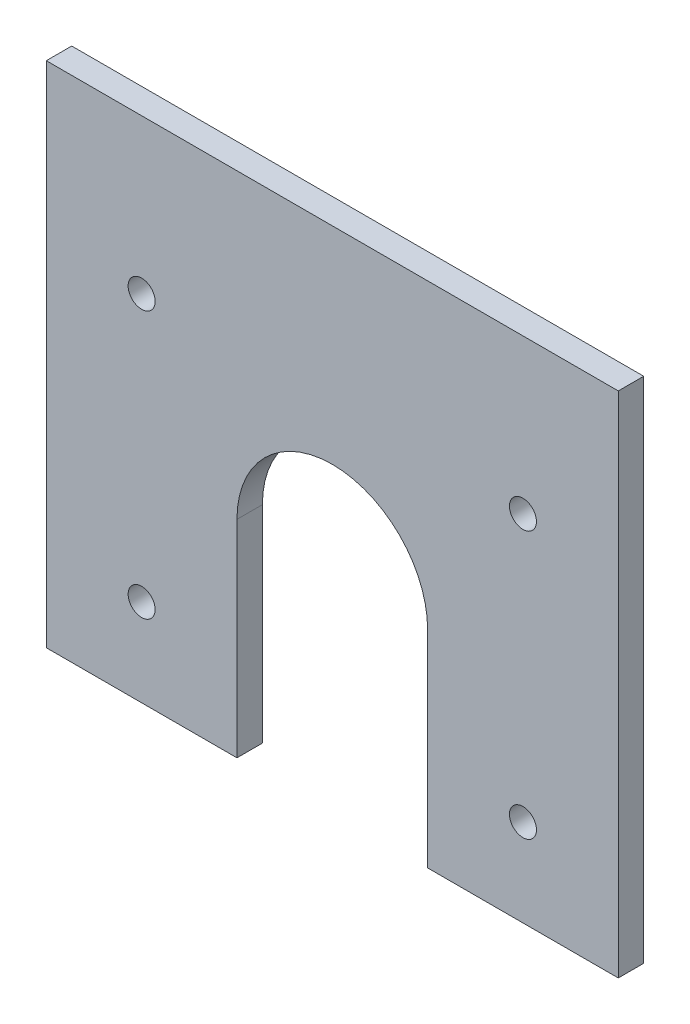
SolidWorks part; units mm, degrees
material "普通碳钢"
ref_plane "Front Plane" through (0, 0, 0) normal (0, 0, 1) x (1, 0, 0)
ref_plane "Top Plane" through (0, 0, 0) normal (0, 1, 0) x (1, 0, 0)
ref_plane "Right Plane" through (0, 0, 0) normal (1, 0, 0) x (0, 0, -1)
sketch "Sketch1" plane through (0, 0, 0) normal (0, 0, 1) x (1, 0, 0)
  line L0 (-180, 160) -> (180, 160)
  line L1 (180, 160) -> (180, -160)
  line L2 (180, -160) -> (-180, -160)
  line L3 (-180, -160) -> (-180, 160)
  point P2 (0, 160)
  point P5 (-180, 0)
  dimension "D1" = 360
  dimension "D2" = 320
extrude "Extrude1" add sketch "Sketch1" along normal mid plane 16
sketch "Sketch2" plane through (0, 0, 8) normal (0, 0, 1) x (1, 0, 0)
  line L0 (-60, -160) -> (-60, -30)
  line L1 (-180, -160) -> (180, -160) construction
  line L2 (60, -160) -> (60, -30)
  line L3 (-60, -160) -> (60, -160)
  arc A0 (-60, -30) -> (60, -30) centre (0, -30) cw
  dimension "D1" = 60
  dimension "D2" = 130
extrude "Extrude2" cut sketch "Sketch2" against normal blind 16
sketch "Sketch3" plane through (0, 0, 8) normal (0, 0, 1) x (1, 0, 0)
  line L0 (-180, -160) -> (-60, -160) construction
  circle A0 centre (-120, 63) radius 8.5
  dimension "D1" = 17
  dimension "D2" = 223
  dimension "D3" = 120
extrude "Extrude3" cut sketch "Sketch3" against normal blind 16
pattern_linear "LPattern1" count 2 spacing 240 along (1, 0, 0) count 2 spacing 168 along (0, -1, 0) of "Extrude3"
